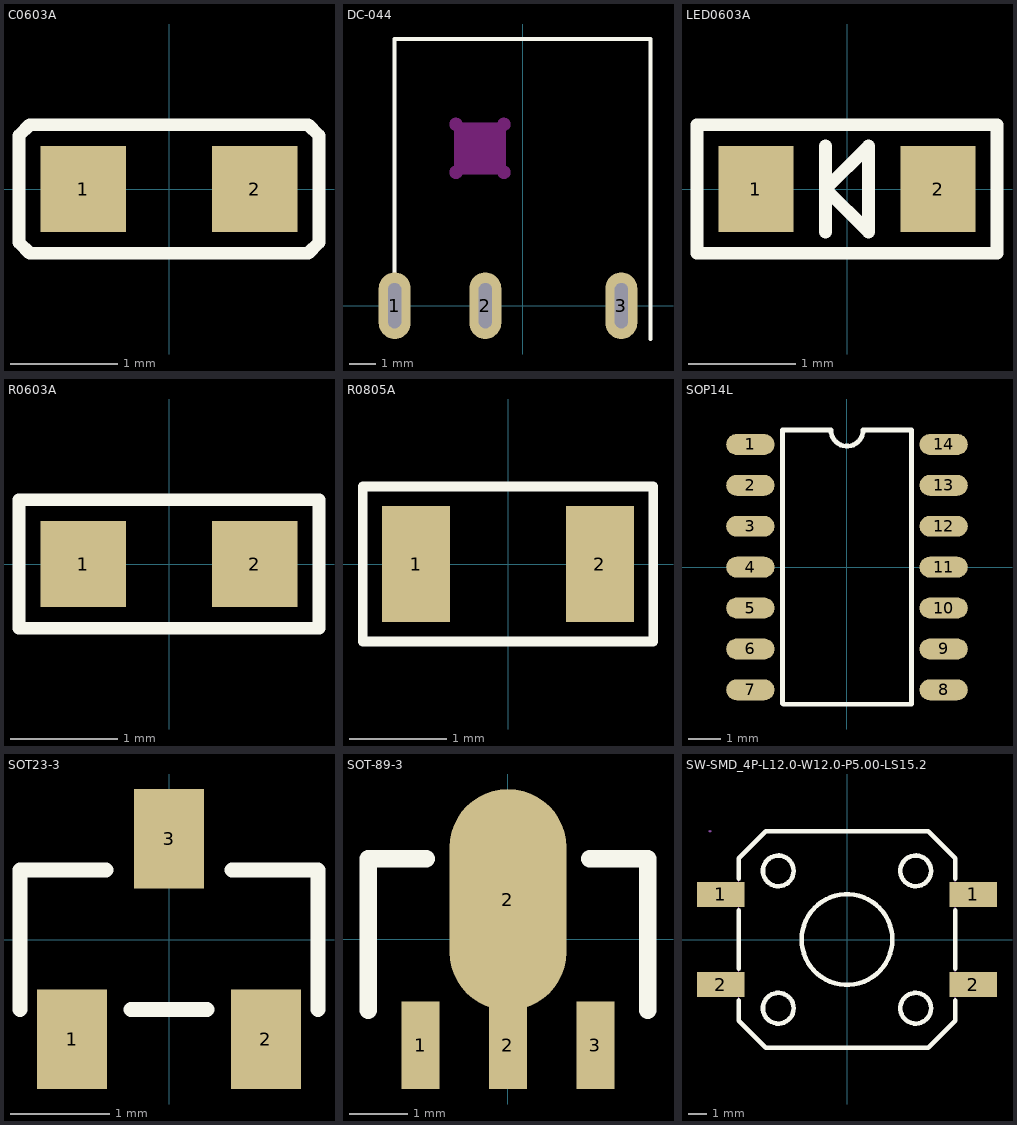
[diagram p0: the footprints below, top view; thin cyan lines are the x and y axes]
# Altium footprint library MISC75799-2.PcbLib: 9 footprints
Each footprint in its own frame and in the unit in brackets; x right, y up, seen from the top. Pads: shape width x height; smd on the part's side, far side on the other; paste and mask are expansions set on the pad; w line width, h text height; cw(c..) or ccw(c..) is an arc to the next point about the centre after c.

## C0603A [mm] "SMD capacitor"
pads (2):
  rect 0.8x0.8 smd mask+0.08: 1(-0.8,0) 2(0.8,0)
Top Overlay:
  lines w0.12: 0.551,-0.6 1.2,-0.6 ; -1.4,-0.5 -1.4,0.5 -1.3,0.6 1.3,0.6 1.4,0.5 1.4,-0.5 1.3,-0.6 -1.3,-0.6 -1.4,-0.5

## DC-044 [mm] "DC power jack through-hole - Yueqing Jinghong"
pads (3):
  oval 1.2x2.5 hole 0.5 slot 1.7 at 90 deg: 1(-4.8,0) 2(-1.4,0) 3(3.7,0)
Top Overlay:
  lines w0.15: -4.8,-1 -4.8,10 4.8,10 4.8,-1.25
Keep-Out Layer:
  board cut-out: -0.7,6.6 -0.74,6.6 -0.813,6.63 -0.87,6.687 -0.9,6.76 -0.9,6.8 -0.9,6.84 -0.87,6.913 -0.813,6.97 -0.74,7 -0.7,7 -0.66,7 -0.587,6.97 -0.53,6.913 -0.5,6.84 -0.5,6.8 -0.5,6.76 -0.53,6.687 -0.587,6.63 -0.66,6.6
  board cut-out: -2.5,4.8 -2.54,4.8 -2.613,4.83 -2.67,4.887 -2.7,4.96 -2.7,5 -2.7,5.04 -2.67,5.113 -2.613,5.17 -2.54,5.2 -2.5,5.2 -2.46,5.2 -2.387,5.17 -2.33,5.113 -2.3,5.04 -2.3,5 -2.3,4.96 -2.33,4.887 -2.387,4.83 -2.46,4.8
  board cut-out: -0.7,4.8 -0.74,4.8 -0.813,4.83 -0.87,4.887 -0.9,4.96 -0.9,5 -0.9,5.04 -0.87,5.113 -0.813,5.17 -0.74,5.2 -0.7,5.2 -0.66,5.2 -0.587,5.17 -0.53,5.113 -0.5,5.04 -0.5,5 -0.5,4.96 -0.53,4.887 -0.587,4.83 -0.66,4.8
  board cut-out: -2.5,6.6 -2.54,6.6 -2.613,6.63 -2.67,6.687 -2.7,6.76 -2.7,6.8 -2.7,6.84 -2.67,6.913 -2.613,6.97 -2.54,7 -2.5,7 -2.46,7 -2.387,6.97 -2.33,6.913 -2.3,6.84 -2.3,6.8 -2.3,6.76 -2.33,6.687 -2.387,6.63 -2.46,6.6
  board cut-out: -2.5,5 -2.5,6.8 -0.7,6.8 -0.7,5
Keep-Out Layer:
  circle w0.1: c-2.5,6.8 r0.2
  circle w0.1: c-0.7,6.8 r0.2
  circle w0.1: c-0.7,5 r0.2
  circle w0.1: c-2.5,5 r0.2
  lines w0.15: -2.5,5 -0.7,5 -0.7,6.8 -2.5,6.8 -2.5,5

## LED0603A [mm] "SMD LED"
pads (2):
  rect 0.7x0.8 smd: 1(-0.85,0) 2(0.85,0)
Top Overlay:
  lines w0.12: -0.2,-0.4 -0.2,0.4 ; -1.4,-0.6 1.4,-0.6 1.4,0.6 -1.4,0.6 -1.4,-0.6 ; -0.2,0 0.2,-0.4 0.2,0.4 -0.2,0

## R0603A [mm] "SMD resistor"
height 0.5
pads (2):
  rect 0.8x0.8 smd mask+0.08: 1(-0.8,0) 2(0.8,0)
Top Overlay:
  lines w0.12: -1.4,-0.6 1.4,-0.6 1.4,0.6 -1.4,0.6 -1.4,-0.6

## R0805A [mm] "SMD resistor"
pads (2):
  rect 0.7x1.2 smd paste+0 mask+0.08: 1(-0.95,0) 2(0.95,0)
Top Overlay:
  lines w0.1: -1.5,-0.8 -1.5,0.8 1.5,0.8 1.5,-0.8 -1.5,-0.8

## SOP14L [mm]
pads (14):
  oval 1.5x0.65 smd: 1(-3,3.81) 2(-3,2.54) 3(-3,1.27) 4(-3,0) 5(-3,-1.27) 6(-3,-2.54) 7(-3,-3.81) 8(3,-3.81) 9(3,-2.54) 10(3,-1.27) 11(3,0) 12(3,1.27) 13(3,2.54) 14(3,3.81)
Top Overlay:
  lines w0.15: 2,-4.255 -1.98,-4.255 -2,-4.235 -2,4.255 -0.5,4.255 ccw(c0,4.255) 0.5,4.255 2,4.255 2,-4.235

## SOT23-3 [mm] "SMD IC/MOS*"
pads (3):
  rect 0.7x1 smd: 1(-0.975,-1) 2(0.975,-1) 3(0,1.016)
Top Overlay:
  lines w0.15: -1.5,-0.7 -1.5,0.7 -0.635,0.7 ; -0.381,-0.7 0.381,-0.7 ; 0.635,0.7 1.5,0.7 1.5,-0.7

## SOT-89-3 [mm] "SMD linear regulator"
pads (4):
  rect 0.65x1.5 smd mask+0.1: 1(-1.5,-1.82) 2(0,-1.82) 3(1.5,-1.82)
  oval 2x3.8 smd mask+0.1: 2(0,0.68)
Top Overlay:
  lines w0.3: -2.4,-1.22 -2.4,1.38 -1.4,1.38 ; 1.4,1.38 2.4,1.38 2.4,-1.22

## SW-SMD_4P-L12.0-W12.0-P5.00-LS15.2 [mm]
pads (4):
  rect 2.64x1.4 smd: 1(-7,2.5) 1(7,2.5) 2(-7,-2.5) 2(7,-2.5)
Top Overlay:
  circle w0.254: c-3.81,-3.81 r0.852
  circle w0.254: c3.81,-3.81 r0.852
  circle w0.254: c3.81,3.81 r0.852
  circle w0.254: c-3.81,3.81 r0.852
  circle w0.254: c0,0 r2.515
  lines w0.254: -6,-3.381 -6,-4.5 -4.5,-6 4.5,-6 6,-4.5 6,-3.381 ; -6,-1.619 -6,1.619 ; -6,3.381 -6,4.5 -4.5,6 4.5,6 6,4.5 6,3.381 ; 6,-1.619 6,1.619
Mechanical 6:
  lines w0.051: -6,-4.5 -6,4.5 -4.5,6 4.5,6 6,4.5 6,-4.5 4.5,-6 -4.5,-6 -6,-4.5
Mechanical 7:
  region: -6.61,-3 -6.61,-2 -5.99,-2 -5.99,-3
  region: -6.61,2 -6.61,3 -5.99,3 -5.99,2
  region: 5.99,-3 5.99,-2 6.61,-2 6.61,-3
  region: 5.99,2 5.99,3 6.61,3 6.61,2
Mechanical 8:
  region: -7.54,6 -7.54,5.975 -7.575,5.94 -7.625,5.94 -7.66,5.975 -7.66,6 -7.66,6.025 -7.625,6.06 -7.575,6.06 -7.54,6.025 -7.54,6
Mechanical 9:
  region: -7.6,-3 -7.6,-2 -6.6,-2 -6.6,-3
  region: -7.6,2 -7.6,3 -6.6,3 -6.6,2
  region: 6.6,-3 6.6,-2 7.6,-2 7.6,-3
  region: 6.6,2 6.6,3 7.6,3 7.6,2